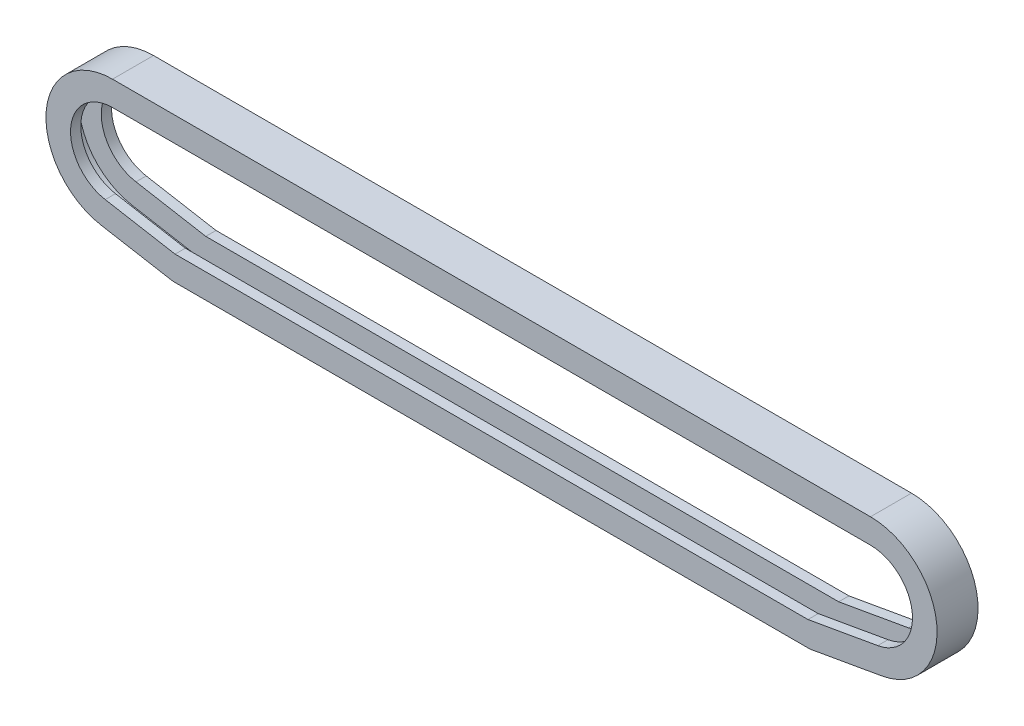
from build123d import *

# Parameters (mm, degrees)
BOSS_EXTRUDE1_DEPTH = 10
CUT_EXTRUDE1_DEPTH  = 5


with BuildPart() as part:
    # Sketch2 → Boss-Extrude1 (new, symmetric)
    with BuildSketch(Plane.XY):
        with BuildLine():
            Line((-185, 32.5), (185, 32.5))
            ThreePointArc((185, 32.5), (217.376327688, 2.832561639), (190.643565774, -32.006251973))
            Line((190.643565774, -32.006251973), (155.524931981, -38.198614636))
            Line((155.524931981, -38.198614636), (-155.524931981, -38.198614636))
            Line((-155.524931981, -38.198614636), (-190.643565774, -32.006251973))
            ThreePointArc((-190.643565774, -32.006251973), (-217.376327688, 2.832561639), (-185, 32.5))
        make_face()
        with BuildLine():
            Line((-185, 20.5), (185, 20.5))
            ThreePointArc((185, 20.5), (205.421991311, 1.786692726), (188.559787642, -20.188558937))
            Line((188.559787642, -20.188558937), (154.475068019, -26.198614636))
            Line((154.475068019, -26.198614636), (-154.475068019, -26.198614636))
            Line((-154.475068019, -26.198614636), (-188.559787642, -20.188558937))
            ThreePointArc((-188.559787642, -20.188558937), (-205.421991311, 1.786692726), (-185, 20.5))
        make_face(mode=Mode.SUBTRACT)
    extrude(amount=BOSS_EXTRUDE1_DEPTH, both=True)

    # Sketch8 → Cut-Extrude1 (cut, symmetric)
    with BuildSketch(Plane.XY):
        with BuildLine():
            Line((155.437443318, -37.198614636), (190.469917597, -31.02144422))
            ThreePointArc((190.469917597, -31.02144422), (216.38013299, 2.745405897), (185, 31.5))
            Line((185, 31.5), (-185, 31.5))
            ThreePointArc((-185, 31.5), (-216.38013299, 2.745405897), (-190.469917597, -31.02144422))
            Line((-190.469917597, -31.02144422), (-155.437443318, -37.198614636))
            Line((-155.437443318, -37.198614636), (155.437443318, -37.198614636))
        make_face()
    extrude(amount=CUT_EXTRUDE1_DEPTH, both=True, mode=Mode.SUBTRACT)


solid = part.part
